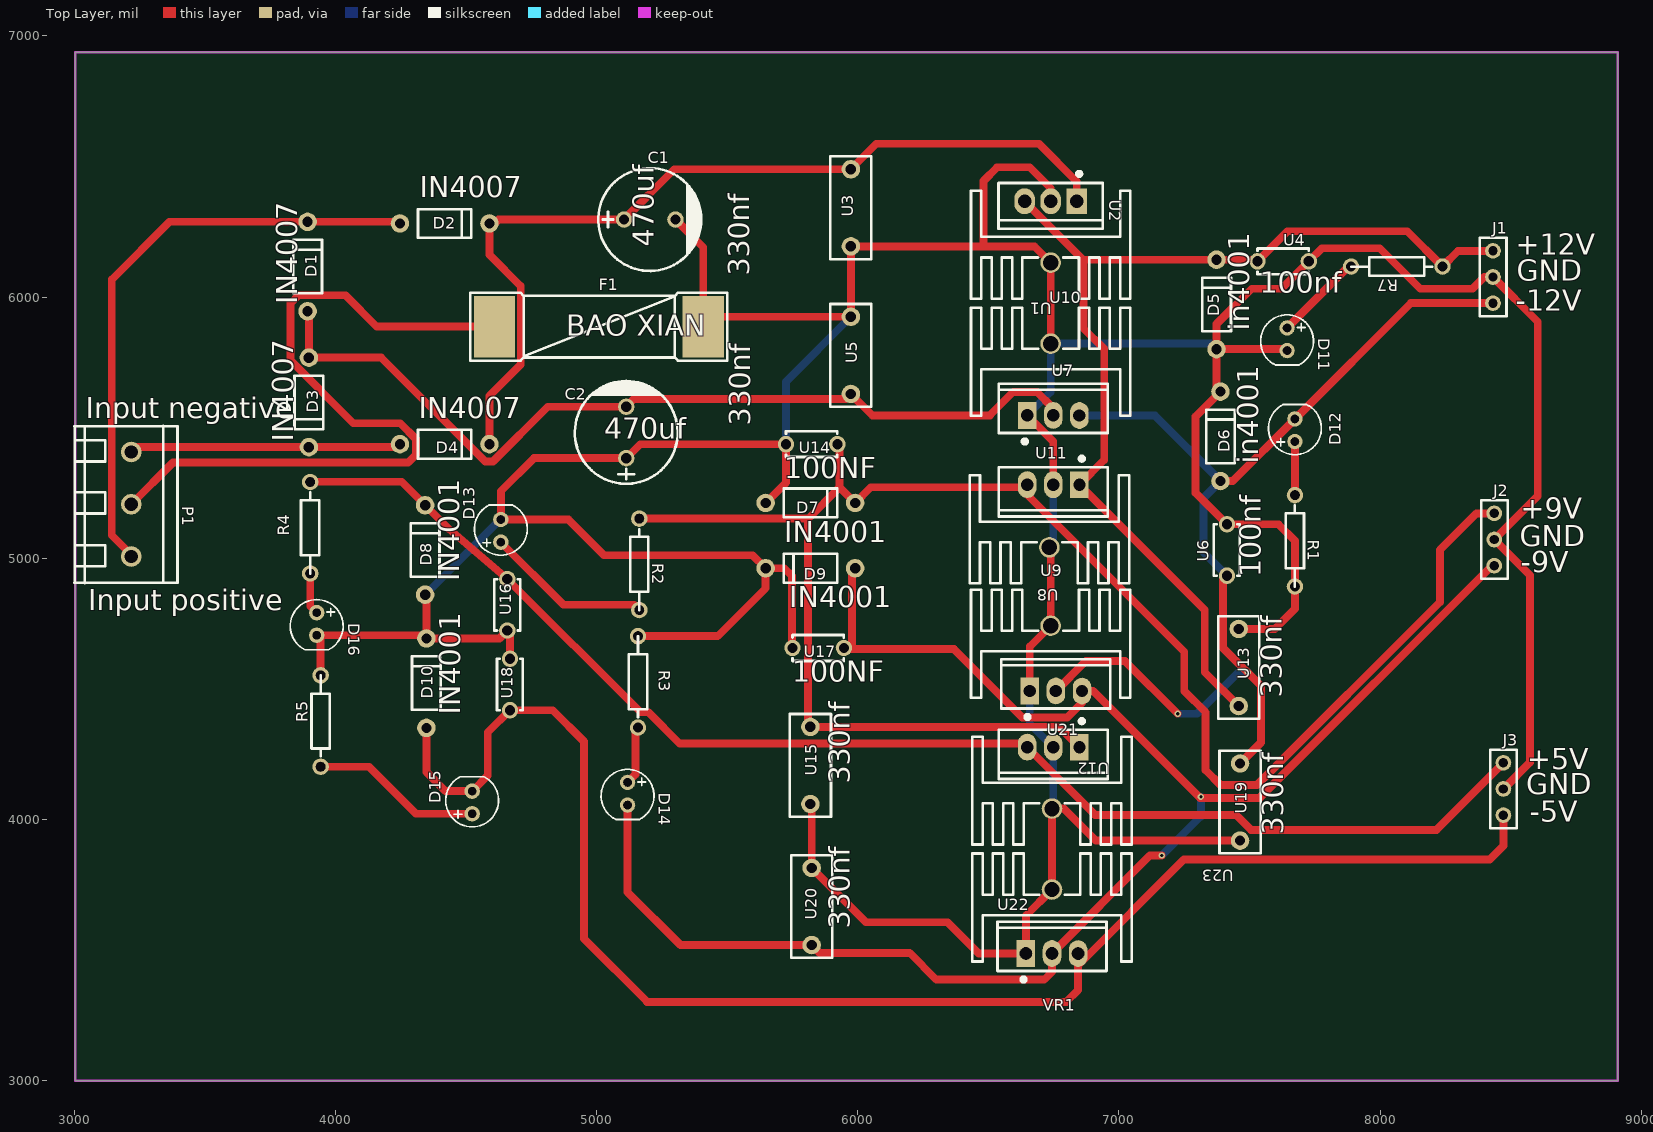
[diagram p0: Top Layer view]
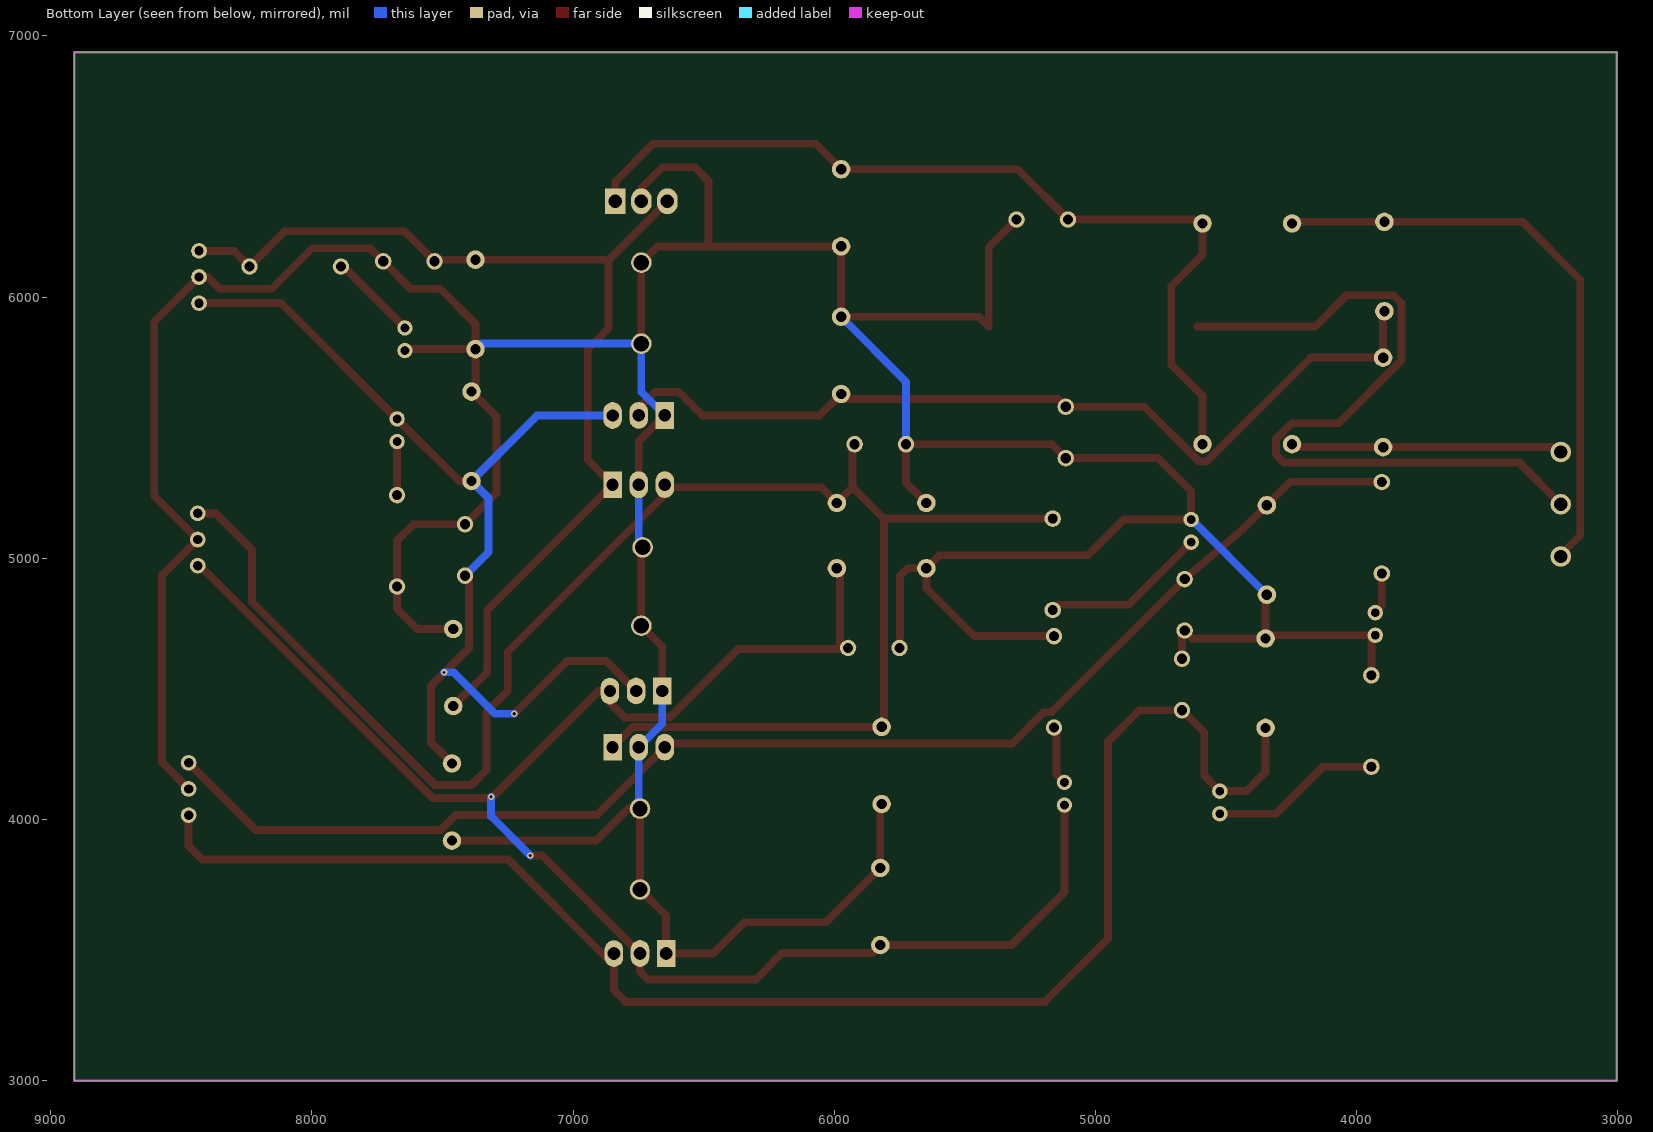
[diagram p1: Bottom Layer view, seen from below]
# Altium PCB MISC51935.pcbdoc
Units mil, origin at the board's own origin, x right, y up, seen from the top; angles counter-clockwise.
Board outline 5905.51 x 3937.01 mil, 2 copper layers (Top Layer, Bottom Layer), stack 0 mil thick; 53 components, 18 nets, 110 pads, 4 vias.

## Layer stack, top to bottom
Top Layer: signal copper (thickness not stored)
Bottom Layer: signal copper (thickness not stored)

## Board outline
3003.9,6937.01 3003.9,3000 8909.41,3000 8909.41,6937.01

## Design rules (kind name [scope] priority, off if disabled: settings)
BoardOutlineClearance Plane_Default_1 [All] p2 off: genericclearance=6 ignorepadtopadclearanceinfootprint=FALSE except(0: Arc-SplitContinuation Track-SplitContinuation SMDPad-SplitContinuation THPad-SplitContinuation Via-SplitContinuation Fill-SplitContinuation Region-SplitContinuation Poly-SplitContinuation Text-SplitContinuation Hole-SplitContinuation; 6: Arc-OutlineEdge Track-OutlineEdge SMDPad-OutlineEdge THPad-OutlineEdge Via-OutlineEdge Fill-OutlineEdge Region-OutlineEdge Poly-OutlineEdge Text-OutlineEdge Hole-OutlineEdge Arc-CutoutEdge Track-CutoutEdge SMDPad-CutoutEdge THPad-CutoutEdge Via-CutoutEdge Fill-CutoutEdge Region-CutoutEdge Poly-CutoutEdge Text-CutoutEdge Hole-CutoutEdge)
BoardOutlineClearance Copper_Default_1 [All] p4 off: genericclearance=6 ignorepadtopadclearanceinfootprint=FALSE except(0: Arc-SplitContinuation Track-SplitContinuation SMDPad-SplitContinuation THPad-SplitContinuation Via-SplitContinuation Fill-SplitContinuation Region-SplitContinuation Poly-SplitContinuation Text-SplitContinuation Hole-SplitContinuation; 6: Arc-OutlineEdge Track-OutlineEdge SMDPad-OutlineEdge THPad-OutlineEdge Via-OutlineEdge Fill-OutlineEdge Region-OutlineEdge Poly-OutlineEdge Text-OutlineEdge Hole-OutlineEdge Arc-CutoutEdge Track-CutoutEdge SMDPad-CutoutEdge THPad-CutoutEdge Via-CutoutEdge Fill-CutoutEdge Region-CutoutEdge Poly-CutoutEdge Text-CutoutEdge Hole-CutoutEdge)
BoardOutlineClearance Copper_gge8332_1 [All] p6 off: genericclearance=6 ignorepadtopadclearanceinfootprint=FALSE except(0: Arc-SplitContinuation Track-SplitContinuation SMDPad-SplitContinuation THPad-SplitContinuation Via-SplitContinuation Fill-SplitContinuation Region-SplitContinuation Poly-SplitContinuation Text-SplitContinuation Hole-SplitContinuation; 6: Arc-OutlineEdge Track-OutlineEdge SMDPad-OutlineEdge THPad-OutlineEdge Via-OutlineEdge Fill-OutlineEdge Region-OutlineEdge Text-OutlineEdge Hole-OutlineEdge Arc-CutoutEdge Track-CutoutEdge SMDPad-CutoutEdge THPad-CutoutEdge Via-CutoutEdge Fill-CutoutEdge Region-CutoutEdge Text-CutoutEdge Hole-CutoutEdge; 10: Poly-OutlineEdge Poly-CutoutEdge)
BoardOutlineClearance Copper_gge8326_1 [All] p8 off: genericclearance=6 ignorepadtopadclearanceinfootprint=FALSE except(0: Arc-SplitContinuation Track-SplitContinuation SMDPad-SplitContinuation THPad-SplitContinuation Via-SplitContinuation Fill-SplitContinuation Region-SplitContinuation Poly-SplitContinuation Text-SplitContinuation Hole-SplitContinuation; 6: Arc-OutlineEdge Track-OutlineEdge SMDPad-OutlineEdge THPad-OutlineEdge Via-OutlineEdge Fill-OutlineEdge Region-OutlineEdge Text-OutlineEdge Hole-OutlineEdge Arc-CutoutEdge Track-CutoutEdge SMDPad-CutoutEdge THPad-CutoutEdge Via-CutoutEdge Fill-CutoutEdge Region-CutoutEdge Text-CutoutEdge Hole-CutoutEdge; 10: Poly-OutlineEdge Poly-CutoutEdge)
BoardOutlineClearance Default_1 [All] p10: genericclearance=6 ignorepadtopadclearanceinfootprint=FALSE except(0: Arc-SplitContinuation Track-SplitContinuation SMDPad-SplitContinuation THPad-SplitContinuation Via-SplitContinuation Fill-SplitContinuation Region-SplitContinuation Poly-SplitContinuation Text-SplitContinuation Hole-SplitContinuation; 6: Arc-OutlineEdge Track-OutlineEdge SMDPad-OutlineEdge THPad-OutlineEdge Via-OutlineEdge Fill-OutlineEdge Region-OutlineEdge Poly-OutlineEdge Text-OutlineEdge Hole-OutlineEdge Arc-CutoutEdge Track-CutoutEdge SMDPad-CutoutEdge THPad-CutoutEdge Via-CutoutEdge Fill-CutoutEdge Region-CutoutEdge Poly-CutoutEdge Text-CutoutEdge Hole-CutoutEdge)
Clearance Plane_Default [All] p1 off: gap=6 ignorepadtopadclearanceinfootprint=FALSE
Clearance Copper_Default [All] p3 off: gap=6 ignorepadtopadclearanceinfootprint=FALSE
Clearance Copper_gge8332 [All] p5 off: gap=6 ignorepadtopadclearanceinfootprint=FALSE except(10: Poly-Track Poly-SMDPad Poly-THPad Poly-Via Poly-Fill Poly-Region Poly-Poly Poly-Arc Poly-Text Poly-Hole)
Clearance Copper_gge8326 [All] p7 off: gap=6 ignorepadtopadclearanceinfootprint=FALSE except(10: Poly-Track Poly-SMDPad Poly-THPad Poly-Via Poly-Fill Poly-Region Poly-Poly Poly-Arc Poly-Text Poly-Hole)
Clearance Default [All] p9: gap=6 ignorepadtopadclearanceinfootprint=FALSE
DiffPairsRouting differentialPair [All] p1: maxlimit=6 minlimit=6 mostfreqgap=6 toplayer_minwidth=5 toplayer_prefwidth=10 toplayer_maxwidth=100 toplayer_mingap=6 toplayer_prefgap=6 toplayer_maxgap=6 bottomlayer_minwidth=5 bottomlayer_prefwidth=10 bottomlayer_maxwidth=100 bottomlayer_mingap=6 bottomlayer_prefgap=6 bottomlayer_maxgap=6 maxuncoupledlength=10
HoleToHoleClearance otherClearance [All] p1: gap=11.81 allowstackedmicrovias=TRUE
Length netLength [All] p1: minlimit=0 maxlimit=0
MatchedLengths netLengthTolerance [All] p1: tolerance=1000
PasteMaskExpansion Common [All] p1: expansion=0
PlaneConnect Default_4 [All] p1: planeconnectstyle=Relief reliefexpansion=20 reliefentries=4 reliefconductorwidth=0 reliefairgap=10
PolygonConnect gge8332 [All] p1 off: connectstyle=Relief reliefconductorwidth=0 reliefentries=4 polygonreliefangle="90 Angle" airgapwidth=1 smdpad.connectstyle=Relief smdpad.reliefconductorwidth=0 smdpad.reliefentries=4 smdpad.polygonreliefangle="90 Angle" smdpad.airgapwidth=10 via.connectstyle=Relief via.reliefconductorwidth=10 via.reliefentries=4 via.polygonreliefangle="90 Angle" via.airgapwidth=10
PolygonConnect gge8326 [All] p2 off: connectstyle=Relief reliefconductorwidth=0 reliefentries=4 polygonreliefangle="90 Angle" airgapwidth=1 smdpad.connectstyle=Relief smdpad.reliefconductorwidth=0 smdpad.reliefentries=4 smdpad.polygonreliefangle="90 Angle" smdpad.airgapwidth=10 via.connectstyle=Relief via.reliefconductorwidth=10 via.reliefentries=4 via.polygonreliefangle="90 Angle" via.airgapwidth=10
PolygonConnect Default_5 [All] p3: connectstyle=Relief reliefconductorwidth=0 reliefentries=4 polygonreliefangle="90 Angle" airgapwidth=1 smdpad.connectstyle=Relief smdpad.reliefconductorwidth=0 smdpad.reliefentries=4 smdpad.polygonreliefangle="90 Angle" smdpad.airgapwidth=10 via.connectstyle=Relief via.reliefconductorwidth=10 via.reliefentries=4 via.polygonreliefangle="90 Angle" via.airgapwidth=10
RoutingVias Default_3 [All] p1: holewidth=12 width=24 viastyle="Through Hole" minholewidth=12 minwidth=24 maxholewidth=2362 maxwidth=3938
SolderMaskExpansion Common_1 [IsVia] p1: expansion=-1000 istentingtop=TRUE
SolderMaskExpansion Common_1 [All] p2: expansion=2 istentingtop=FALSE
Width Default_2 [All] p1: maxlimit=10 minlimit=10 preferedwidth=10 toplayer_minwidth=30 toplayer_maxwidth=1000 toplayer_prefwidth=30 bottomlayer_minwidth=30 bottomlayer_maxwidth=1000 bottomlayer_prefwidth=30

## Components (designator, comment, footprint, x,y, rotation, side; value= is the part's Value field where it differs from the comment)
C1 "470uF" CAP-TH_BD10.0-P5.00-D0.6-FD 5203.9,6297.01 r0 top
C2 "470uF" CAP-TH_BD10.0-P5.00-D0.6-FD 5113.9,5482.01 r90 top
D1 "1N4007" DO-41_BD2.4-L4.7-P8.70-D0.9-RD 3893.9,6117.01 r270 top
D2 "1N4007" DO-41_BD2.4-L4.7-P8.70-D0.9-RD 4418.9,6282.01 r180 top
D3 "1N4007" DO-41_BD2.4-L4.7-P8.70-D0.9-RD 3898.9,5597.01 r90 top
D4 "1N4007" DO-41_BD2.4-L4.7-P8.70-D0.9-RD 4418.9,5437.01 r180 top
D5 "IN4001" DO-41_BD2.4-L4.7-P8.70-D0.9-RD 7373.9,5972.01 r270 top
D6 "IN4001" DO-41_BD2.4-L4.7-P8.70-D0.9-RD 7388.9,5467.01 r270 top
D7 "IN4001" DO-41_BD2.4-L4.7-P8.70-D0.9-RD 5818.9,5212.01 r180 top
D8 "IN4001" DO-41_BD2.4-L4.7-P8.70-D0.9-RD 4343.9,5032.01 r270 top
D9 "IN4001" DO-41_BD2.4-L4.7-P8.70-D0.9-RD 5818.9,4962.01 r0 top
D10 "IN4001" DO-41_BD2.4-L4.7-P8.70-D0.9-RD 4348.9,4522.01 r270 top
D11 "Red" 发光二极管 7643.9,5882.01 r270 top
D12 "Red" 发光二极管 7673.9,5447.01 r90 top
D13 "Red" 发光二极管 4633.9,5062.01 r90 top
D14 "Red" 发光二极管 5118.9,4142.01 r270 top
D15 "Red" 发光二极管 4523.9,4022.01 r90 top
D16 "Red" 发光二极管 3928.9,4792.01 r270 top
F1 "10A" FUSE-SMD_5-20MM 5008.9,5887.01 r0 top
J1 "1*3 pin header" 1*3排针 8438.9,6072.01 r0 top
J2 "1*3 pin header" 1*3排针 8443.9,5067.01 r0 top
J3 "1*3 pin header" 1*3排针 8478.9,4112.01 r0 top
P1 "WJ500V-5.08-3P" CONN-TH_3P-P5.00_WJ500V-5.08-3P 3218.9,5207.01 r270 top
R1 "10k 1/4W" "10K直插电阻 PCB封装" 7673.9,5072.01 r270 top
R2 "10k 1/4W" "10K直插电阻 PCB封装" 5163.9,4982.01 r270 top
R3 "10k 1/4W" "10K直插电阻 PCB封装" 5158.9,4522.01 r90 top
R4 "10k 1/4W" "10K直插电阻 PCB封装" 3903.9,5122.01 r270 top
R5 "10k 1/4W" "10K直插电阻 PCB封装" 3943.9,4372.01 r90 top
R7 "10k 1/4W" "10K直插电阻 PCB封装" 8068.9,6117.01 r180 top
U1 "15*10.5*21" SINK-TH_L15.0-W10.5-H21.0 6738.9,6132.01 r180 top
U2 "L7812CV" TO-220-3_L10.0-W4.5-P2.54-T 6738.9,6367.01 r270 top
U3 "330nF" CAP-TH_L10.0-W4.0-P7.50-D0.6-1 5973.9,6342.01 r90 top
U4 "100NF" CAP-TH_L5.0-W2.5-P5.00-D1.0 7628.9,6137.01 r0 top
U5 "330nF" CAP-TH_L10.0-W4.0-P7.50-D0.6-1 5973.9,5777.01 r90 top
U6 "100NF" CAP-TH_L5.0-W2.5-P5.00-D1.0 7413.9,5032.01 r270 top
U7 "L7912CV" TO-220-3_L10.0-W4.5-P2.54-L#1 6748.9,5547.01 r0 top
U8 "15*10.5*21" SINK-TH_L15.0-W10.5-H21.0 6733.9,5042.01 r180 top
U9 "15*10.5*21" SINK-TH_L15.0-W10.5-H21.0 6738.9,4742.01 r0 top
U10 "15*10.5*21" SINK-TH_L15.0-W10.5-H21.0 6738.9,5822.01 r0 top
U11 "L7809CV" TO-220-3_L10.0-W4.5-P2.54-L#1 6748.9,5282.01 r180 top
U12 "L7805CV-DG" TO-220-3_L10.0-W4.5-P2.54-L#1 6748.9,4277.01 r180 top
U13 "330nF" CAP-TH_L10.0-W4.0-P7.50-D0.6-1 7458.9,4582.01 r270 top
U14 "100NF" CAP-TH_L5.0-W2.5-P5.00-D1.0 5823.9,5437.01 r180 top
U15 "330nF" CAP-TH_L10.0-W4.0-P7.50-D0.6-1 5818.9,4207.01 r90 top
U16 "100NF" CAP-TH_L5.0-W2.5-P5.00-D1.0 4658.9,4822.01 r270 top
U17 "100NF" CAP-TH_L5.0-W2.5-P5.00-D1.0 5848.9,4657.01 r0 top
U18 "100NF" CAP-TH_L5.0-W2.5-P5.00-D1.0 4668.9,4517.01 r270 top
U19 "330nF" CAP-TH_L10.0-W4.0-P7.50-D0.6-1 7463.9,4067.01 r270 top
U20 "330nF" CAP-TH_L10.0-W4.0-P7.50-D0.6-1 5823.9,3667.01 r90 top
U21 "LM7909CT" TO-220-3_L10.0-W4.5-P2.54-L#1 6758.9,4492.01 r0 top
U22 "15*10.5*21" SINK-TH_L15.0-W10.5-H21.0 6743.9,3732.01 r0 top
U23 "15*10.5*21" SINK-TH_L15.0-W10.5-H21.0 6743.9,4042.01 r180 top
VR1 "L7905" TO-220-3_L10.0-W4.5-P2.54-L#2 6743.9,3487.01 r0 top

## Footprints (in the part's own frame and the unit in brackets; to place one, negate y for a bottom-side part, rotate by r counter-clockwise, add the part's x,y. Pads: shape width x height; smd on the part's side, far side on the other; paste and mask are expansions set on the pad)
1*3排针 [mil]
  round 60 hole 36 paste+0 mask+2: 1(-6.68,-95) 2(-6.68,5) 3(-6.68,105)
  silkscreen extent -57,-145 45,155
"10K直插电阻 PCB封装" [mm]
  round 1.6 hole 0.92 slot 0.925 at 0 deg paste+0 mask+0.051: 1(-4.318,0) 2(4.572,0)
  silkscreen extent -3.3,-0.89 4.57,0.89
CAP-TH_BD10.0-P5.00-D0.6-FD [mm]
  round 1.6 hole 1 copper offset 0,0 paste+0 mask+0.05: 1(-2.5,0)
  round 1.6 hole 1 paste+0 mask+0.05: 2(2.5,0)
  silkscreen extent -5,-5 5.08,5
CAP-TH_L5.0-W2.5-P5.00-D1.0 [mm]
  round 1.6 hole 1 paste+0 mask+0.051: 1(-2.5,0) 2(2.5,0)
  silkscreen extent -2.5,-1.27 2.5,1.25
CAP-TH_L10.0-W4.0-P7.50-D0.6-1 [mm]
  round 1.8 hole 1 paste+0 mask+0.051: 1(-3.75,0) 2(3.75,0)
  silkscreen extent -5,-2 5,2
CONN-TH_3P-P5.00_WJ500V-5.08-3P [mm]
  round 2 hole 1.3 paste+0 mask+0.051: 1(-5.08,0) 2(0,0) 3(5.08,0)
  silkscreen extent -7.64,-5.53 7.66,4.5
DO-41_BD2.4-L4.7-P8.70-D0.9-RD [mm]
  round 1.8 hole 1 paste+0 mask+0.051: 1(-4.35,0) 2(4.35,0)
  silkscreen extent -2.6,-1.4 2.6,1.4
FUSE-SMD_5-20MM [mm]
  rect 4x6 smd paste+0 mask+0.051: 1(-10.16,0) 2(10.16,0)
  silkscreen extent -12.5,-3.3 12.5,3.3
SINK-TH_L15.0-W10.5-H21.0 [mm]
  round 2 hole 1.5 paste+0 mask+0.051: 1(0,0)
  silkscreen extent -7.75,-7 7.75,3.5
TO-220-3_L10.0-W4.5-P2.54-L#1 [mm]
  rect 1.8x2.6 hole 1.2 paste+0 mask+0.051: 1(-2.54,0.005)
  oval 1.8x2.6 hole 1.2 paste+0 mask+0.051: 2(0,0.005)
  oval 1.8x2.6 hole 1.2 copper offset 0,0 paste+0 mask+0.051: 3(2.54,-0.005)
  silkscreen extent -5.3,-2.73 5.3,3.09
TO-220-3_L10.0-W4.5-P2.54-L#2 [mm]
  rect 1.8x2.6 hole 1.2 slot 1.205 at 90 deg paste+0 mask+0.051: 1(-2.54,0.005)
  oval 1.8x2.6 hole 1.2 slot 1.205 at 90 deg paste+0 mask+0.051: 2(0,0.005) 3(2.54,-0.005)
  silkscreen extent -5.3,-2.73 5.3,3.09
TO-220-3_L10.0-W4.5-P2.54-T [mm]
  rect 2.5x2 hole 1.3 paste+0 mask+0.051: 1(0,2.54)
  oval 2.5x2 hole 1.3 paste+0 mask+0.051: 2(0,0) 3(0,-2.54)
  silkscreen extent -2.86,-5.08 2.67,5.08
发光二极管 [mil]
  round 59.06 hole 31.5 slot 31.7 at 0 deg paste+0 mask+2: 1(0,0) 2(86.61,0)
  silkscreen extent -50,-101 142,101

## Via types
v1: diameter 24.02, hole 12, Top Layer to Bottom Layer, 4 vias

## Nets (pads, with @x,y where several pads share a name; then routed paths per layer and width w, separated by ;. In a path a pad name is that pad's centre, name@x,y a point inside that pad or via, vN(x,y) a via of type N, cw(c..) or ccw(c..) an arc to the next point about the centre after c; other vN are vias at no path point)
C1_1: C1.1 D2.1 D4.1 U2.1 U3.2 | length 3454.5
  Top Layer w30: D4.1 4590.16,5622.01 4710.16,5742.01 4710.16,6042.01 4590.16,6162.01 D2.1 4610.48,6282.01 4625.48,6297.01 C1.1 5298.12,6489.65 U3.2 6071.26,6587.01 6693.9,6587.01 6838.9,6442.01 U2.1
C2_2: C2.2 D1.2 D3.2 U5.1 U7.2 | length 3425.8
  Top Layer w30: D1.2 3898.9,5940.75 D3.2 4176.06,5768.27 4573.9,5370.43 4603.9,5370.43 4813.9,5580.43 C2.2 5143.9,5610.43 5953.9,5610.43 U5.1 6056.07,5547.2 6506.07,5547.2 6596.07,5637.2 6686.07,5637.2 6746.07,5577.2 6746.07,5550.03 U7.2
D2_2: D1.1 D2.2 P1.3 | length 2289
  Top Layer w30: P1.3 3218.9,5013.27 3143.9,5088.27 3143.9,6067.01 3365.16,6288.27 D1.1 4241.38,6288.27 D2.2
D4_2: D3.1 D4.2 P1.1 | length 1040.8
  Top Layer w30: P1.1 3238.9,5425.75 D3.1 4228.9,5425.75 4240.16,5437.01 D4.2
GND: C1.2 C2.1 D5.2 D6.1 D7.2 D8.2 D9.1 D10.1 D11.2 D13.2 D16.2 F1.2 J1.2 J2.2 J3.2 R1.2 R3.2 R5.2 U1.1 U2.2 U3.1 U4.2 U5.2 U6.1 U7.1 U8.1 U9.1 U10.1 U11.2 U12.2 U13.1 U14.2 U15.1 U16.2 U17.1 U18.1 U19.2 U20.2 U21.1 U22.1 U23.1 VR1.1 | length 19400.1
  Top Layer w30: R5.2 3943.9,4690.4 D16.2 4336.77,4705.4 D10.1 ; D8.2 4348.9,4855.75 D10.1 ; U18.1 4668.9,4713.58 U16.2 4628.59,4693.27 D10.1 ; R3.2 5463.9,4702.01 5647.64,4885.75 D9.1 ; C1.2 5408.9,6190.43 F1.2 5446.54,5924.65 U5.2 U3.1 6481.42,6194.37 ; D7.2 5725.47,5289.84 U14.2 5167.32,5437.01 C2.1 4760.48,5383.59 4633.9,5257.01 D13.2 4892.29,5148.62 5028.9,5012.01 5597.64,5012.01 D9.1 ; U17.1 5748.9,4658.59 5748.9,4932.01 5718.9,4962.01 D9.1 ; U15.1 5823.9,4054.37 U20.2 6031.54,3607.01 6343.9,3607.01 6463.71,3487.2 VR1.1 6643.9,3632.01 U22.1 U23.1 6788.9,4042.01 6911.54,3919.37 U19.2 ; U7.1 6748.9,5447.21 U11.2 ; U21.1 6658.9,4662.01 U9.1 6738.9,5037.01 U8.1 ; U10.1 U1.1 6676.54,6194.37 6481.42,6194.37 ; U2.2 6738.9,6417.01 6658.9,6497.01 6533.9,6497.01 6481.42,6444.53 6481.42,6194.37 ; U13.1 7596.54,4729.65 7673.9,4807.01 R1.2 7673.9,5067.01 7610.48,5130.43 U6.1 7293.9,5250.43 7293.9,5543.27 D6.1 7373.9,5653.27 D5.2 ; D11.2 7638.55,5800.75 D5.2 ; J3.2 8573.9,4218.69 8573.9,4935.33 J2.2 8603.9,5238.69 8603.9,5905.33 J1.2 8398.9,6077.01 8353.9,6032.01 8153.9,6032.01 7998.9,6187.01 7777.33,6187.01 U4.2 7622.33,6032.01 7508.9,6032.01 7373.9,5897.01 D5.2
  Bottom Layer w30: D8.2 4631.77,5148.62 D13.2 ; U14.2 5725.47,5676.22 U5.2 ; U7.1 6738.9,5637.21 U10.1 7352.64,5822.01 D5.2 ; U21.1 6658.9,4366.82 U12.2 6748.9,4047.01 U23.1 ; U8.1 6748.9,5057.01 U11.2
P1_2: F1.1 P1.2 | length 2895.1
  Top Layer w30: P1.2 3378.9,5367.01 4278.9,5367.01 4308.9,5397.01 4308.9,5457.01 4248.9,5517.01 4068.9,5517.01 3828.9,5757.01 3828.9,5977.01 3858.9,6007.01 4038.9,6007.01 4158.9,5887.01 F1.1
R1_1: D12.1 R1.1 | length 205
  Top Layer w30: R1.1 D12.1
R2_2: D13.1 R2.2 | length 637.7
  Top Layer w30: D13.1 4873.9,4822.01 5143.9,4822.01 R2.2
R3_1: D14.1 R3.1 | length 226.6
  Top Layer w30: D14.1 5148.9,4172.01 5148.9,4342.01 R3.1
R4_2: D16.1 R4.2 | length 160.4
  Top Layer w30: R4.2 3903.9,4817.01 D16.1
R5_1: D15.1 R5.1 | length 654.6
  Top Layer w30: R5.1 4128.9,4202.01 4308.9,4022.01 D15.1
R7_2: D11.1 R7.2 | length 342.3
  Top Layer w30: D11.1 7878.9,6117.01 R7.2
U7_3: D6.2 D12.2 J1.1 U6.2 U7.3 U19.1 U21.2 | length 4146.2
  Top Layer w30: U21.2 6873.71,4607.01 7022.87,4607.01 v1(7225.1,4404.78) ; D6.2 7436.03,5295.75 D12.2 8117.29,5977.01 J1.1 ; U6.2 7398.9,4918.58 7398.9,4657.01 7543.9,4512.01 7543.9,4294.65 U19.1
  Bottom Layer w30: U7.3 7137.84,5546.81 D6.2 7323.9,5230.75 7323.9,5023.58 U6.2 ; v1(7225.1,4404.78) 7298.99,4404.78 7457.73,4563.52 v1(7493.84,4563.52)
U11_1: D5.1 J1.3 R7.1 U2.3 U4.1 U11.1 U13.2 | length 4050.9
  Top Layer w30: U2.3 6862.64,6143.27 6863.9,6143.27 ; U13.2 7328.9,4564.36 7328.9,4801.81 U11.1 6943.9,5376.81 6943.9,5553.27 6943.9,5801.23 6863.9,5881.23 6863.9,6143.27 ; J1.3 8298.9,6177.01 R7.1 8103.9,6252.01 7645.48,6252.01 U4.1 7523.9,6143.27 D5.1 6863.9,6143.27
U12_1: D7.1 J2.3 R2.1 U11.3 U12.1 U14.1 U15.2 | length 6674.8
  Top Layer w30: R2.1 5810.16,5152.01 ; U14.1 5922.32,5429.85 5930.16,5422.01 5930.16,5272.01 ; U11.3 6638.69,5272.01 U11.3@6620.16,5272.01 ; U12.1 6771.06,4354.65 U15.2 5818.9,4363.27 5810.16,4372.01 5810.16,5152.01 ; J2.3 8368.9,5172.01 8228.9,5032.01 8228.9,4832.01 7528.9,4132.01 7388.9,4132.01 7332.03,4188.88 7332.03,4410.14 7250.16,4492.01 7250.16,4642.01 U11.3@6620.16,5272.01 ; 5810.16,5152.01 5930.16,5272.01 ; 5930.16,5272.01 D7.1 6050.16,5272.01 U11.3@6620.16,5272.01
U12_3: D8.1 J3.3 R4.1 U12.3 U16.1 | length 5218.2
  Top Layer w30: R4.1 3923.9,5293.27 4253.9,5293.27 D8.1 4435.7,5111.47 U16.1 5168.9,4410.43 5198.9,4410.43 5318.9,4290.43 6635.66,4290.43 U12.3 6909.09,4017.01 7449.09,4017.01 7505.66,3960.43 7950.27,3960.43 8215.65,3960.43 J3.3
VR1_2: D9.2 D14.2 J2.1 U17.2 U20.1 U21.3 VR1.2 | length 6564
  Top Layer w30: D14.2 5118.9,3722.01 5321.54,3519.37 U20.1 5853.9,3489.37 6198.92,3489.37 6301.28,3387.01 6713.9,3387.01 6743.9,3417.01 VR1.2 7118.71,3862.01 v1(7163.9,3862.01) ; U17.2 5952.13,4652.21 5978.51,4652.21 ; D9.2 5978.51,4952.21 5978.51,4652.21 ; J2.1 8428.31,4972.01 7538.51,4082.21 7310.94,4082.21 6901.34,4491.81 U21.3 6858.91,4447.02 6802.54,4390.65 6630.07,4390.65 6542.61,4478.1 6368.51,4652.21 5978.51,4652.21
  Bottom Layer w30: v1(7163.9,3862.01) 7313.9,4012.01 v1(7313.9,4087.01)
VR1_3: D10.2 D15.2 J3.1 U18.2 VR1.3 | length 5917.8
  Top Layer w30: D10.2 4348.9,4182.01 4422.29,4108.62 D15.2 4583.9,4168.62 4583.9,4333.58 U18.2 4832.33,4418.58 4952.09,4298.82 4952.09,3543.82 5193.9,3302.01 5929.22,3302.01 6643.84,3302.01 6798.9,3302.01 6843.9,3347.01 VR1.3@6843.9,3442.01 ; VR1.3 VR1.3@6843.9,3442.01 ; J3.1 8472.22,3899.32 8419.7,3846.81 7349.15,3846.81 7248.7,3846.81 VR1.3@6843.9,3442.01

## Keep-outs
Board Outline Layer:
  the board outline again, w10

## Silkscreen, mask and mechanical layers (free items; w line width, h text height)
Top Silkscreen Layer:
  text "IN4007" at 4323.9,6382.01 h80
  text "470uf" at 5218.9,6192.01 h80 r90
  text "+12V" at 8518.9,6162.01 h80
  text "330nf" at 5583.9,6082.01 h80 r90
  text "GND" at 8523.9,6062.01 h80
  text "100nf" at 7538.9,6017.01 h80
  text "IN4007" at 3853.9,5972.01 h80 r90
  text "-12V" at 8518.9,5947.01 h80
  text "in4001" at 7498.9,5872.01 h80 r90
  text "BAO XIAN" at 4883.9,5852.01 h80
  text "Input negative" at 3043.9,5537.01 h80
  text "IN4007" at 4318.9,5537.01 h80
  text "330nf" at 5588.9,5507.01 h80 r90
  text "470uf" at 5028.9,5457.01 h80
  text "IN4007" at 3838.9,5447.01 h80 r90
  text "in4001" at 7533.9,5362.01 h80 r90
  text "100NF" at 5718.9,5307.01 h80
  text "+9V" at 8538.9,5152.01 h80
  text "IN4001" at 5718.9,5062.01 h80
  text "GND" at 8533.9,5047.01 h80
  text "-9V" at 8538.9,4947.01 h80
  text "100nf" at 7543.9,4927.01 h80 r90
  text "IN4001" at 4473.9,4912.01 h80 r90
  text "IN4001" at 5738.9,4812.01 h80
  text "Input positive" at 3053.9,4802.01 h80
  text "100NF" at 5748.9,4527.01 h80
  text "330nf" at 7623.9,4467.01 h80 r90
  text "IN4001" at 4478.9,4402.01 h80 r90
  text "+5V" at 8563.9,4192.01 h80
  text "330nf" at 5968.9,4137.01 h80 r90
  text "GND" at 8558.9,4097.01 h80
  text "-5V" at 8573.9,3992.01 h80
  text "330nf" at 7628.9,3942.01 h80 r90
  text "330nf" at 5968.9,3582.01 h80 r90